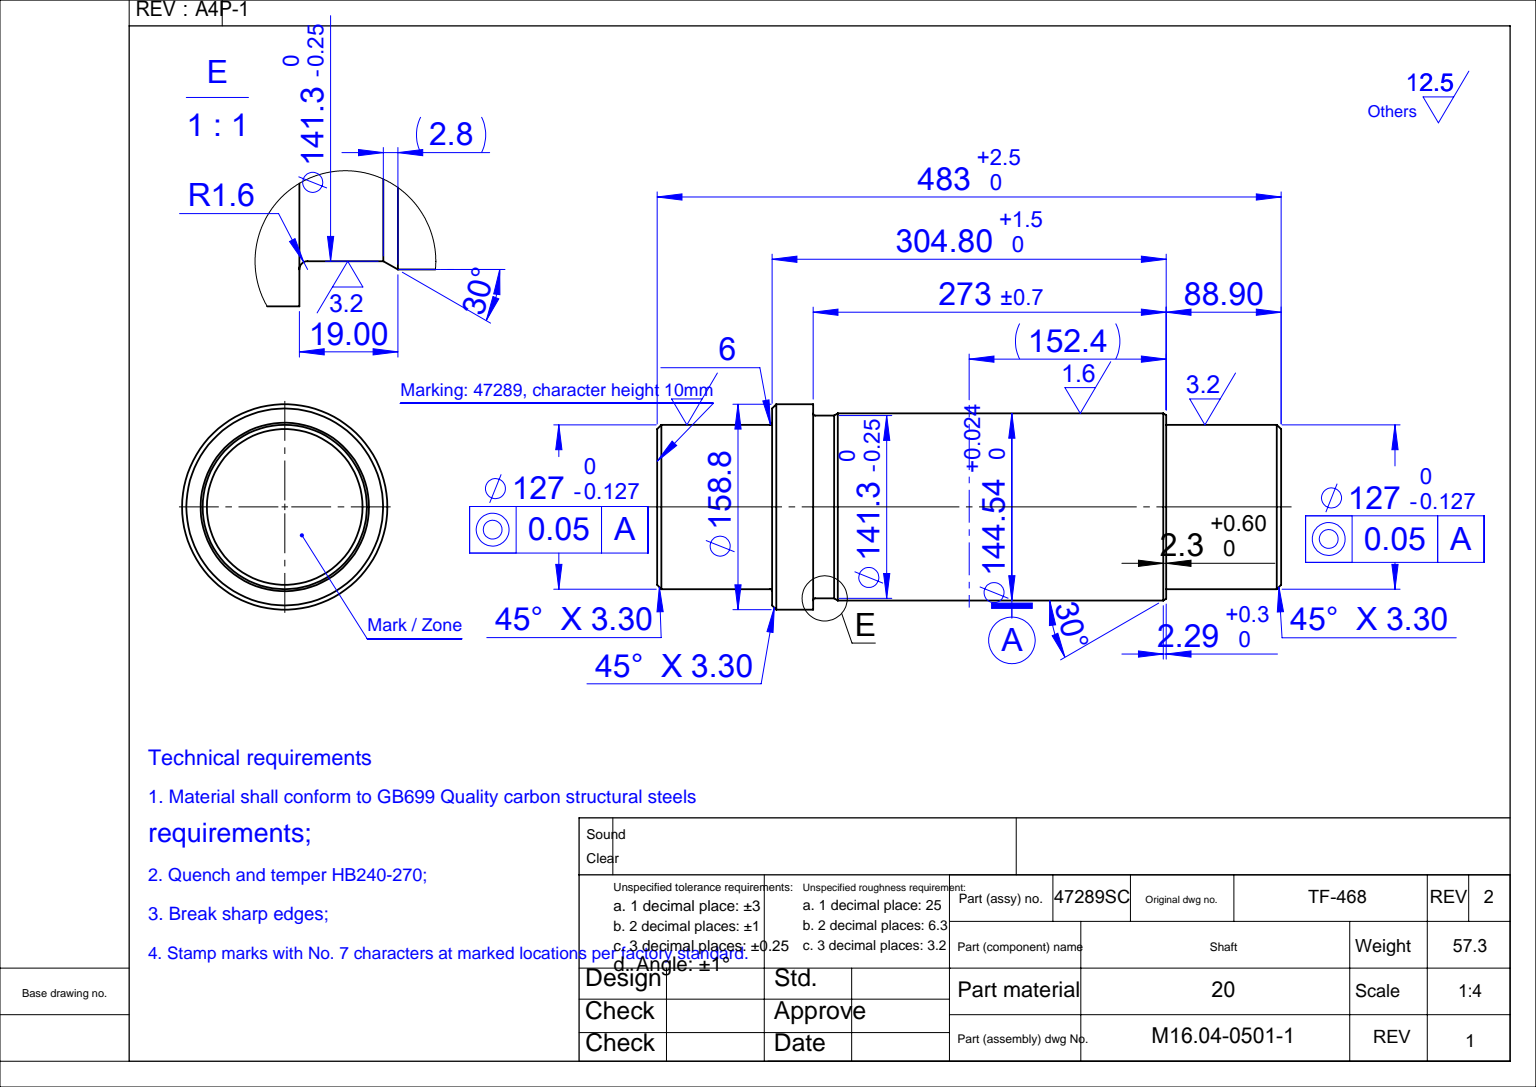
SolidWorks part; units mm, degrees
material "20"
ref_plane "Front Plane" through (0, 0, 0) normal (0, 0, 1) x (1, 0, 0)
ref_plane "Top Plane" through (0, 0, 0) normal (0, 1, 0) x (1, 0, 0)
ref_plane "Right Plane" through (0, 0, 0) normal (1, 0, 0) x (0, 0, -1)
sketch "Sketch1" plane through (0, 0, 0) normal (1, 0, 0) x (0, 0, -1)
  line L0 (-264.5789, 0) -> (259.3234, 0) construction
  line L1 (-237.998, 63.5) -> (-153.9875, 63.5)
  line L2 (-152.4, 65.0875) -> (-152.4, 76.073)
  line L3 (-149.098, 79.375) -> (-120.65, 79.375)
  line L4 (-120.65, 79.375) -> (-120.65, 72.2376)
  line L5 (-119.0625, 70.6501) -> (-104.4046, 70.6501)
  line L6 (-104.4046, 70.6501) -> (-101.6, 72.2694)
  line L7 (-101.6, 72.2694) -> (150.114, 72.2694)
  line L8 (152.4, 70.9495) -> (152.4, 63.5)
  line L9 (152.4, 63.5) -> (237.998, 63.5)
  line L10 (241.3, 60.198) -> (241.3, 0)
  line L11 (-241.3, 60.198) -> (-241.3, 0)
  line L13 (-241.3, 0) -> (241.3, 0)
  line L14 (-152.4, 76.073) -> (-149.098, 79.375)
  line L15 (-241.3, 60.198) -> (-237.998, 63.5)
  line L16 (237.998, 63.5) -> (241.3, 60.198)
  line L17 (150.114, 72.2694) -> (152.4, 70.9495)
  arc A0 (-120.65, 72.2376) -> (-119.0625, 70.6501) centre (-119.0625, 72.2376) ccw
  arc A1 (-153.9875, 63.5) -> (-152.4, 65.0875) centre (-153.9875, 65.0875) ccw
  point P3 (-241.3, 63.5)
  point P6 (-152.4, 79.375)
  point P13 (241.3, 63.5)
  dimension "D10" = 1.5875
  dimension "D20" = 1.5875
  dimension "D1" = 482.6
  dimension "D2" = 88.9
  dimension "D3" = 304.8
  dimension "D4" = 30
  dimension "D5" = 273.05
  dimension "D6" = 158.75
  dimension "D7" = 144.5387
  dimension "D8" = 127
  dimension "D9" = 141.3002
  dimension "D11" = 19.05
  dimension "D12" = 3.302
  dimension "D13" = 45
  dimension "D14" = 3.302
  dimension "D15" = 45
  dimension "D16" = 3.302
  dimension "D17" = 45
  dimension "D18" = 30
  dimension "D19" = 2.286
  dimension "D21" = 152.4
revolve "Revolve1" add sketch "Sketch1" angle 360 about L0
